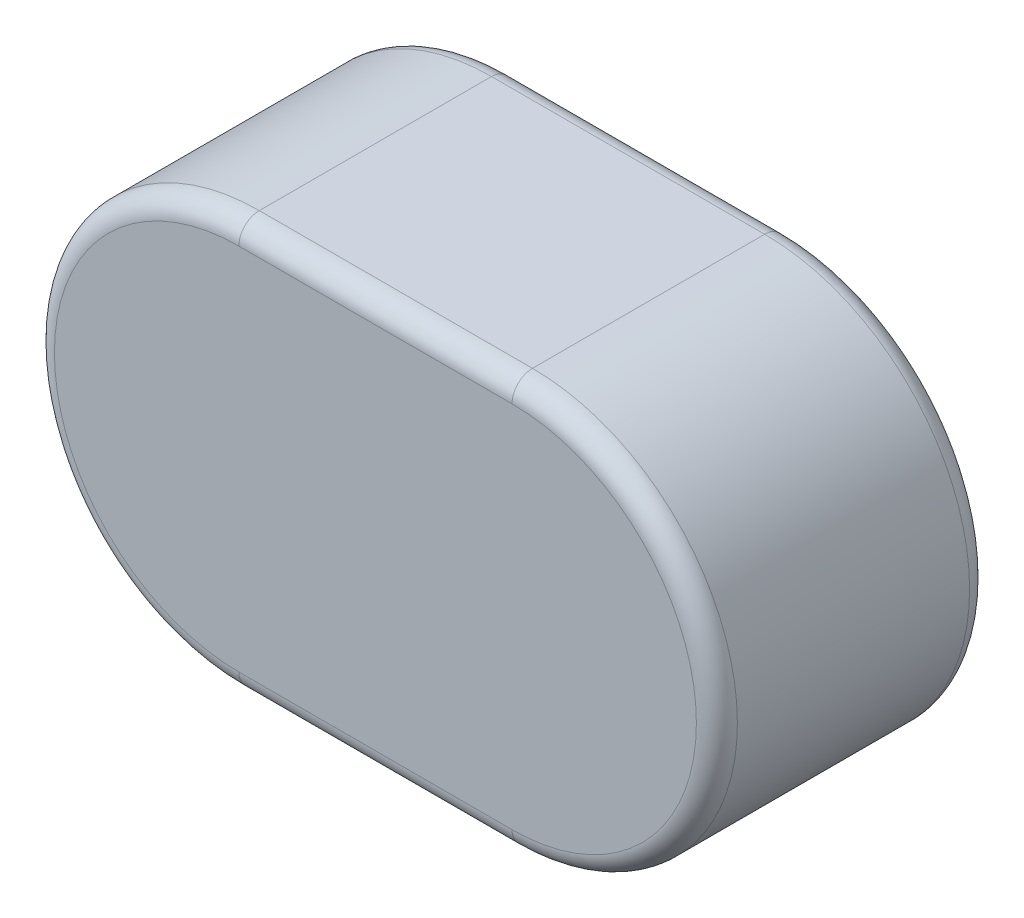
from build123d import *

# Parameters (mm, degrees)
EXTRUDE_523_DEPTH = 8
FILLET_1_R        = 0.6


with BuildPart() as part:
    # 草图1 → Extrude 523 (new body)
    with BuildSketch(Plane.XY):
        with BuildLine():
            Line((-4, 6), (4, 6))
            ThreePointArc((4, 6), (10, 0), (4, -6))
            Line((4, -6), (-4, -6))
            ThreePointArc((-4, -6), (-10, 0), (-4, 6))
        make_face()
    extrude(amount=EXTRUDE_523_DEPTH)

    # 圆角1
    fillet_1_edges = [part.edges().sort_by_distance(p)[0] for p in [
        (10, 0, 8),
        (0, 6, 8),
        (-10, 0, 8),
        (0, 6, 0),
        (10, 0, 0),
        (0, -6, 0),
        (-10, 0, 0),
        (0, -6, 8),
    ]]
    fillet(fillet_1_edges, radius=FILLET_1_R)


solid = part.part
